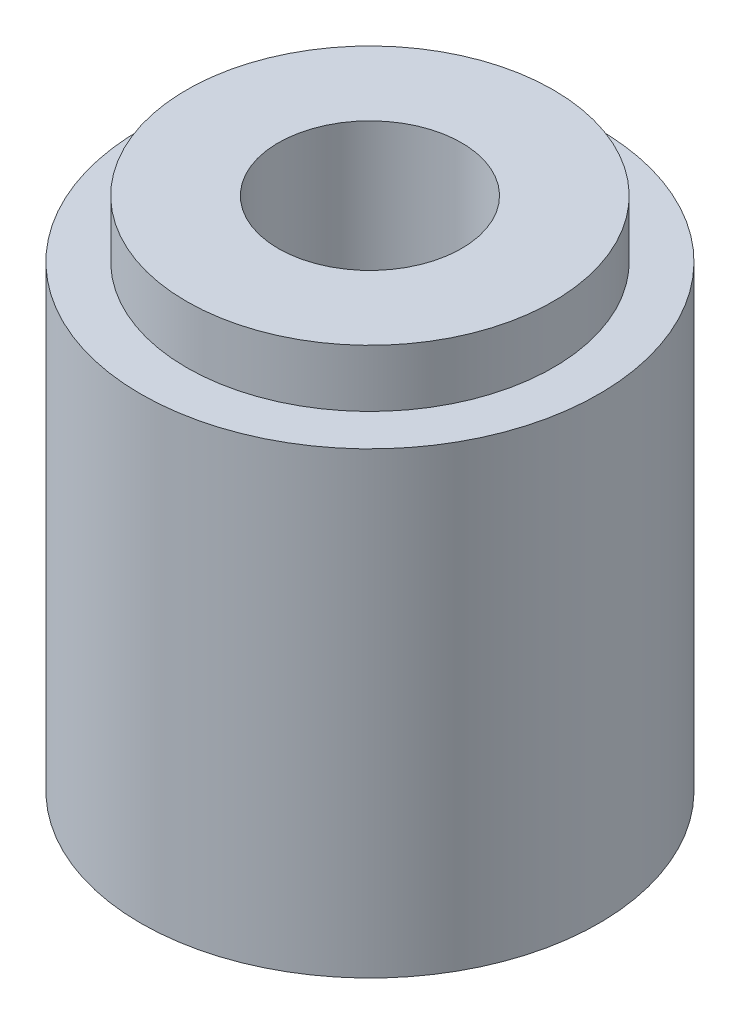
SolidWorks part; units mm, degrees
material "35#"
ref_plane "Front Plane" through (0, 0, 0) normal (0, 0, 1) x (1, 0, 0)
ref_plane "Top Plane" through (0, 0, 0) normal (0, 1, 0) x (1, 0, 0)
ref_plane "Right Plane" through (0, 0, 0) normal (1, 0, 0) x (0, 0, -1)
sketch "Sketch1" plane through (0, 0, 0) normal (0, 0, 1) x (1, 0, 0)
  line L0 (10.25, 0) -> (20, 0)
  line L1 (20, 0) -> (20, 40)
  line L2 (20, 40) -> (16, 40)
  line L3 (16, 40) -> (16, 45)
  line L4 (16, 45) -> (8, 45)
  line L5 (0, 45) -> (0, 0) construction
  line L6 (0, 0) -> (0, 45) construction
  line L7 (8, 45) -> (8, 31.299)
  line L8 (8, 31.299) -> (10.25, 30)
  line L9 (10.25, 30) -> (10.25, 0)
  dimension "D1" = 40
  dimension "D2" = 5
  dimension "D3" = 40
  dimension "D4" = 32
  dimension "D5" = 16
  dimension "D6" = 20.5
  dimension "D7" = 30
  dimension "D8" = 60
revolve "Revolve1" add sketch "Sketch1" angle 360 about L5
cosmetic thread "Cosmetic Thread1" parameters "D1"=18.5, "D2"=26.441
chamfer "Chamfer1" distance 3 angle 45 1 edges at (0, 0, 10.25)
